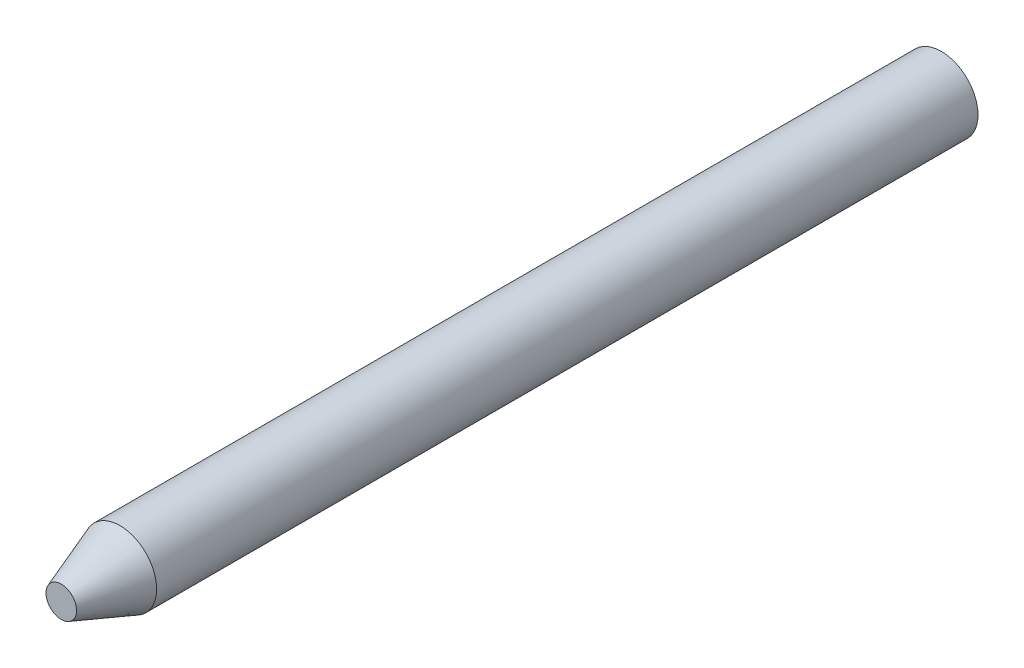
SolidWorks part; units mm, degrees
ref_plane "前视基准面" through (0, 0, 0) normal (0, 0, 1) x (1, 0, 0)
ref_plane "上视基准面" through (0, 0, 0) normal (0, 1, 0) x (1, 0, 0)
ref_plane "右视基准面" through (0, 0, 0) normal (1, 0, 0) x (0, 0, -1)
sketch "草图1" plane through (0, 0, 0) normal (0, 0, 1) x (1, 0, 0)
  circle A0 centre (0, 0) radius 1.25
  dimension "D1" = 2.5
extrude "凸台-拉伸1" add sketch "草图1" along normal blind 30
chamfer "倒角1" distance 2 angle 20 1 edges at (1.25, 0, 30)
